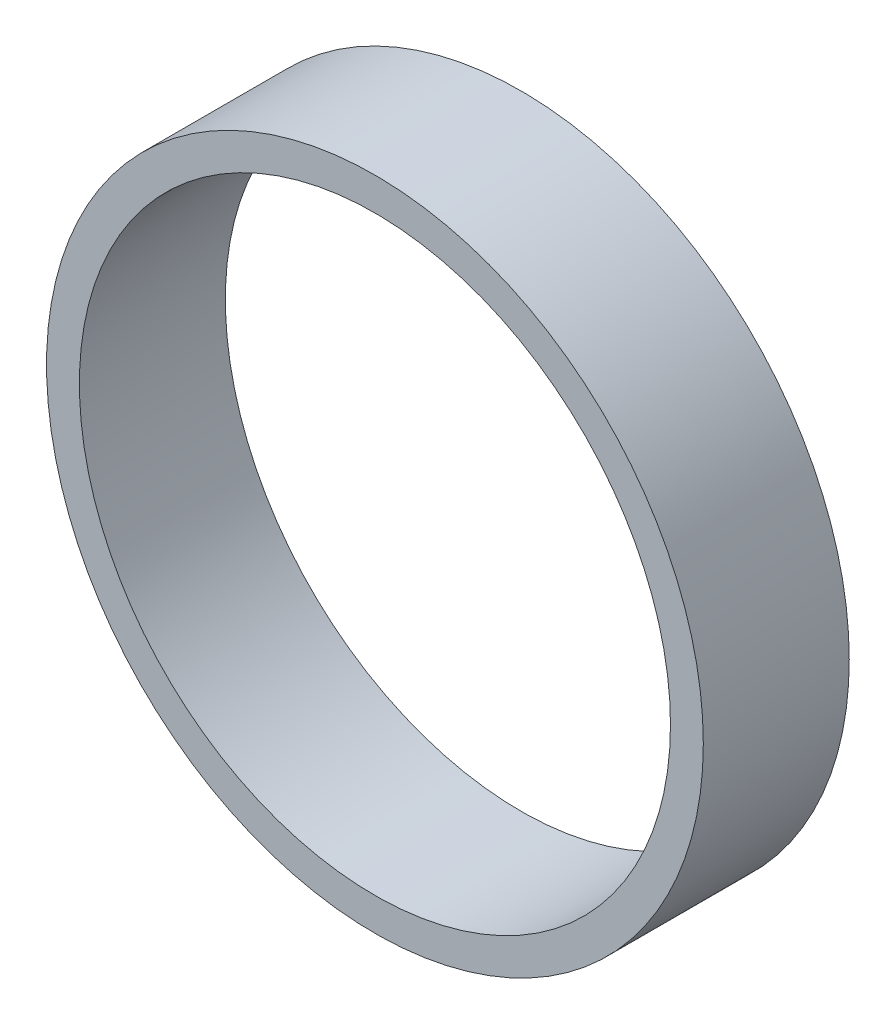
SolidWorks part; units mm, degrees
ref_plane "前视基准面" through (0, 0, 0) normal (0, 0, 1) x (1, 0, 0)
ref_plane "上视基准面" through (0, 0, 0) normal (0, 1, 0) x (1, 0, 0)
ref_plane "右视基准面" through (0, 0, 0) normal (1, 0, 0) x (0, 0, -1)
sketch "草图1" plane through (0, 0, 0) normal (0, 0, 1) x (1, 0, 0)
  circle A0 centre (0, 0) radius 20.25
  circle A1 centre (0, 0) radius 22.5
  dimension "D1" = 40.5
  dimension "D2" = 45
extrude "凸台-拉伸1" add sketch "草图1" along normal blind 10
